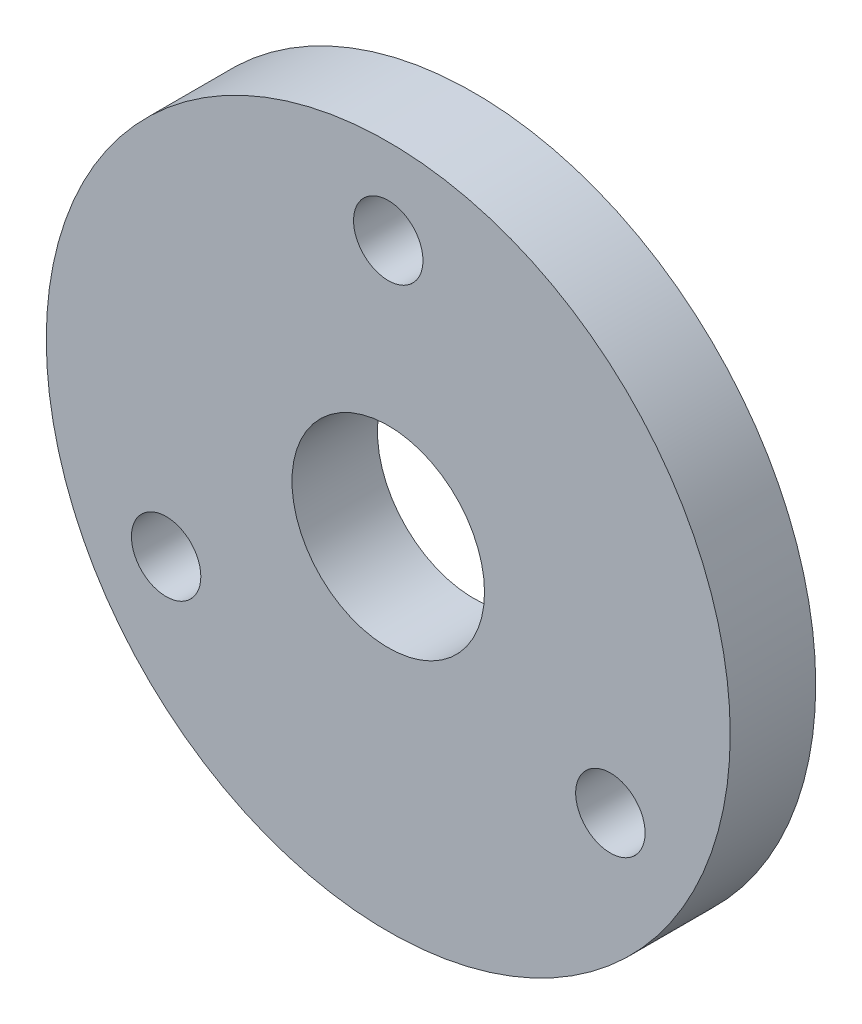
from build123d import *

# Parameters (mm, degrees)
SKETCH1_R           = 25.4
SKETCH1_R_2         = 7.1501
BOSS_EXTRUDE1_DEPTH = 6.35
SKETCH2_R           = 2.5781
CUT_EXTRUDE1_DEPTH  = 6.35


with BuildPart() as part:
    # Sketch1 → Boss-Extrude1 (new body)
    with BuildSketch(Plane.XY):
        Circle(SKETCH1_R)
        Circle(SKETCH1_R_2, mode=Mode.SUBTRACT)
    extrude(amount=-BOSS_EXTRUDE1_DEPTH)

    # Sketch2 → Cut-Extrude1 (cut)
    with BuildSketch(Plane.XY):
        with Locations((0, 19.05)):
            Circle(SKETCH2_R)
        with Locations((16.497783942, -9.525)):
            Circle(SKETCH2_R)
        with Locations((-16.497783942, -9.525)):
            Circle(SKETCH2_R)
    extrude(amount=-CUT_EXTRUDE1_DEPTH, mode=Mode.SUBTRACT)


solid = part.part
